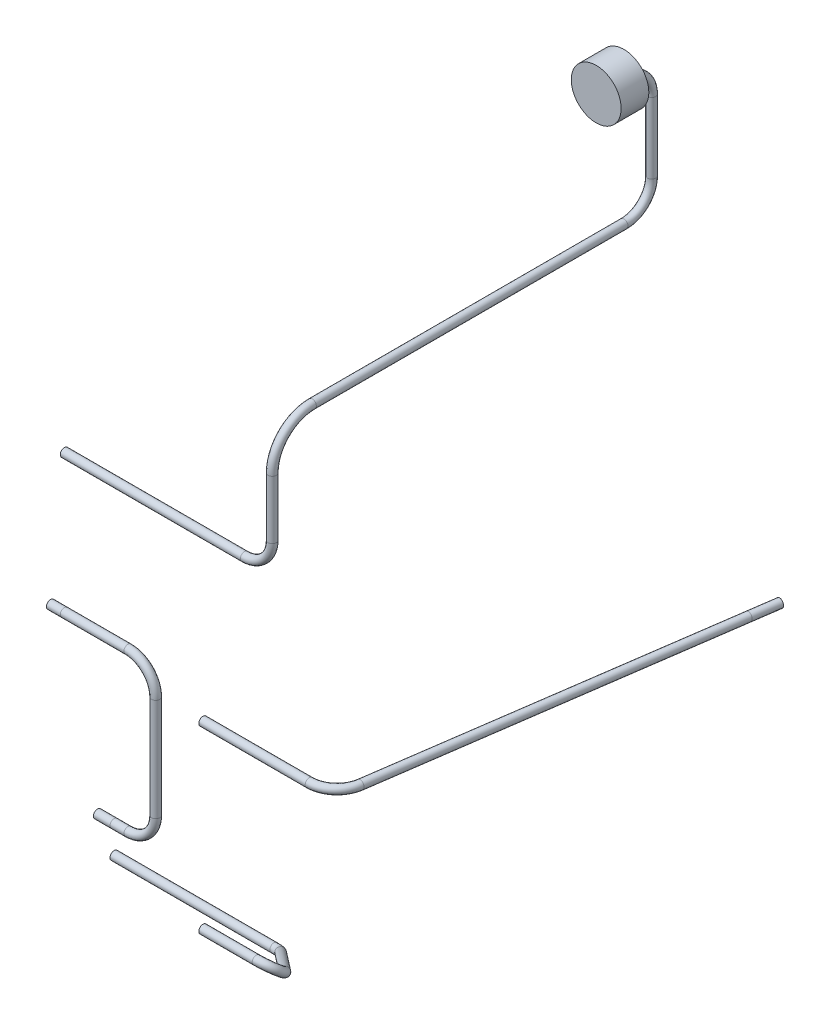
SolidWorks part; units mm, degrees
ref_plane "Front Plane" through (0, 0, 0) normal (0, 0, 1) x (1, 0, 0)
ref_plane "Top Plane" through (0, 0, 0) normal (0, 1, 0) x (1, 0, 0)
ref_plane "Right Plane" through (0, 0, 0) normal (1, 0, 0) x (0, 0, -1)
sketch "Sketch1" plane through (0, -434, 0) normal (0, -1, 0) x (-1, 0, 0)
  line L0 (365.77, 406.0904) -> (367.1842, 396.1909)
  line L1 (364.2851, 405.8783) -> (367.2549, 406.3026) construction
  line L2 (362.2345, 395.4838) -> (372.134, 396.898) construction
  line L3 (367.1842, 396.1909) -> (384.6992, 273.5858)
  line L4 (433, 265) -> (394.5987, 265)
  line L5 (433, 276.5) -> (433, 253.5) construction
  arc A0 (394.5987, 265) -> (384.6992, 273.5858) centre (394.5987, 275) cw
  dimension "D1" = 10
sketch "Sketch2" plane through (0, 0, -297) normal (0, 0, -1) x (-1, 0, 0)
  line L0 (515, -457) -> (492.05, -457)
  line L1 (515, -454.5) -> (515, -459.5) construction
  line L2 (482.05, -467) -> (482.05, -504)
  line L3 (497.05, -514) -> (492.05, -514)
  line L4 (497.05, -511.5) -> (497.05, -516.5) construction
  line L5 (515, -457) -> (520, -457)
  line L6 (520, -465) -> (520, -399) construction
  line L7 (497.05, -514) -> (503.05, -514)
  line L8 (503.05, -535.5) -> (503.05, -504) construction
  arc A0 (482.05, -467) -> (492.05, -457) centre (492.05, -467) cw
  arc A1 (482.05, -504) -> (492.05, -514) centre (492.05, -504) ccw
  point P18 (482.05, -514)
  dimension "D2" = 10
  dimension "D1" = 15
sketch "Sketch3" plane through (0, -524, 0) normal (0, -1, 0) x (-1, 0, 0)
  line L0 (497.05, 297) -> (503.05, 297)
  line L1 (497.05, 299.5) -> (497.05, 294.5) construction
  line L2 (503.05, 294.75) -> (503.05, 405.75) construction
  line L3 (497.05, 297) -> (437.05, 297)
  dimension "D1" = 60
sketch "Sketch4" plane through (0, 0, -265) normal (0, 0, -1) x (-1, 0, 0)
  line L0 (433, -499) -> (403, -499)
  line L1 (433, -487.5) -> (433, -510.5) construction
  dimension "D1" = 30
sketch3d "3DSketch1"
  line L0 (-403, -499, -265) -> (-437.05, -524, -297)
  line L1 (-403, -499, -265) -> (-437.05, -524, -297) construction
  line L2 (-403, -499, -265) -> (-437.05, -524, -297)
sketch3d "3DSketch2"
  line L0 (-433, -499, -265) -> (-403, -499, -265) construction
  line L1 (-497.05, -524, -297) -> (-437.05, -524, -297) construction
  line L2 (-403, -499, -265) -> (-437.05, -524, -297) construction
  line L3 (-433, -499, -265) -> (-413.7177, -499, -265)
  line L4 (-497.05, -524, -297) -> (-439.3826, -524, -297)
  line L5 (-409.8863, -504.056, -271.4717) -> (-435.5513, -522.8996, -295.5915)
  arc A0 (-435.5513, -522.8996, -295.5915) -> (-439.3826, -524, -297) centre (-439.3826, -520.9218, -293.0599) ccw
  arc A1 (-413.7177, -499, -265) -> (-409.8863, -504.056, -271.4717) centre (-413.7177, -502.0782, -268.9401) ccw
  point P6 (-437.05, -524, -297)
  point P8 (-439.3826, -516.9817, -296.1381)
  point P11 (-403, -499, -265)
  point P13 (-413.7177, -498.1381, -272.0183)
  dimension "D1" = 5
sweep "Sweep1" add path "3DSketch2" circular profile diameter 3 parameters "D3"=3
sweep "Sweep2" add path "Sketch2" circular profile diameter 3 parameters "D3"=3
sweep "Sweep3" add path "Sketch1" circular profile diameter 3 parameters "D3"=3
sketch "Sketch41" plane through (0, 0, -297) normal (0, 0, -1) x (-1, 0, 0)
  line L0 (515, -407) -> (520, -407)
  line L1 (515, -404.5) -> (515, -409.5) construction
  line L2 (520, -465) -> (520, -399) construction
  line L3 (515, -407) -> (450, -407)
  line L4 (440, -361.5) -> (440, -397)
  line L5 (440, -361.5) -> (470.5508, -361.5) construction
  arc A0 (450, -407) -> (440, -397) centre (450, -397) cw
  dimension "D1" = 10
sketch "Sketch42" plane through (-440, 0, 0) normal (-1, 0, 0) x (0, 0, 1)
  line L0 (-413.95, -316) -> (-423.95, -316)
  line L1 (-413.95, -304) -> (-413.95, -328) construction
  line L2 (-433.95, -326) -> (-433.95, -351.5)
  line L3 (-423.95, -361.5) -> (-297, -361.5)
  arc A0 (-433.95, -351.5) -> (-423.95, -361.5) centre (-423.95, -351.5) ccw
  arc A1 (-433.95, -326) -> (-423.95, -316) centre (-423.95, -326) cw
  point P12 (-433.95, -316)
  dimension "D2" = 10
  dimension "D1" = 20
sketch3d "3DSketch3"
  line L0 (-515, -407, -297) -> (-450, -407, -297) construction
  line L1 (-440, -361.5, -297) -> (-440, -397, -297) construction
  line L2 (-440, -361.5, -423.95) -> (-440, -361.5, -297) construction
  line L3 (-440, -326, -433.95) -> (-440, -351.5, -433.95) construction
  line L4 (-440, -316, -413.95) -> (-440, -316, -423.95) construction
  line L5 (-515, -407, -297) -> (-450, -407, -297)
  line L6 (-440, -375.9381, -297) -> (-440, -397, -297)
  line L7 (-440, -361.5, -423.95) -> (-440, -361.5, -311.4381)
  line L8 (-440, -326, -433.95) -> (-440, -351.5, -433.95)
  line L9 (-440, -316, -413.95) -> (-440, -316, -423.95)
  arc A0 (-450, -407, -297) -> (-440, -397, -297) centre (-450, -397, -297) ccw construction
  arc A1 (-440, -351.5, -433.95) -> (-440, -361.5, -423.95) centre (-440, -351.5, -423.95) ccw construction
  arc A2 (-440, -326, -433.95) -> (-440, -316, -423.95) centre (-440, -326, -423.95) ccw construction
  arc A3 (-450, -407, -297) -> (-440, -397, -297) centre (-450, -397, -297) ccw
  arc A4 (-440, -351.5, -433.95) -> (-440, -361.5, -423.95) centre (-440, -351.5, -423.95) ccw
  arc A5 (-440, -326, -433.95) -> (-440, -316, -423.95) centre (-440, -326, -423.95) ccw
  arc A6 (-440, -375.9381, -297) -> (-440, -361.5, -311.4381) centre (-440, -375.9381, -311.4381) ccw
  point P5 (-450, -397, -287)
  point P6 (-450, -351.5, -423.95)
  point P7 (-450, -397, -287)
  point P9 (-430, -326, -423.95)
  point P13 (-450, -351.5, -423.95)
  point P17 (-440, -361.5, -297)
  point P19 (-430, -326, -423.95)
  point P22 (-454.4381, -375.9381, -311.4381)
  dimension "D1" = 14.4381
sweep "Sweep4" add path "3DSketch3" circular profile diameter 3 parameters "D3"=3
sketch "Sketch55" plane through (0, 0, -413.95) normal (0, 0, 1) x (1, 0, 0)
  circle A0 centre (-440, -316) radius 9
  dimension "D1" = 18
extrude "Boss-Extrude1" add sketch "Sketch55" against normal blind 10
